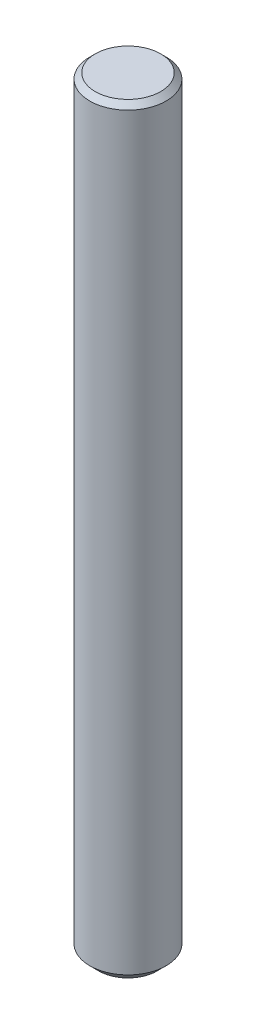
from build123d import *

# Parameters (mm, degrees)
SKETCH2_R           = 21
BOSS_EXTRUDE1_DEPTH = 420
CHAMFER1_SIZE       = 5
CHAMFER2_SIZE       = 3


with BuildPart() as part:
    # Sketch2 → Boss-Extrude1 (new body)
    with BuildSketch(Plane(origin=(0, 0, 0), x_dir=(1, 0, 0), z_dir=(0, 1, 0))):
        with Locations(Location((0, 0, 0), (0, 0, 270))):
            Circle(SKETCH2_R)
    extrude(amount=BOSS_EXTRUDE1_DEPTH)

    # Chamfer1
    chamfer1_edges = [part.edges().sort_by_distance(p)[0] for p in [
        (0, 0, -21),
    ]]
    chamfer(chamfer1_edges, length=CHAMFER1_SIZE)

    # Chamfer2
    chamfer2_edges = [part.edges().sort_by_distance(p)[0] for p in [
        (0, 420, -21),
    ]]
    chamfer(chamfer2_edges, length=CHAMFER2_SIZE)


solid = part.part
